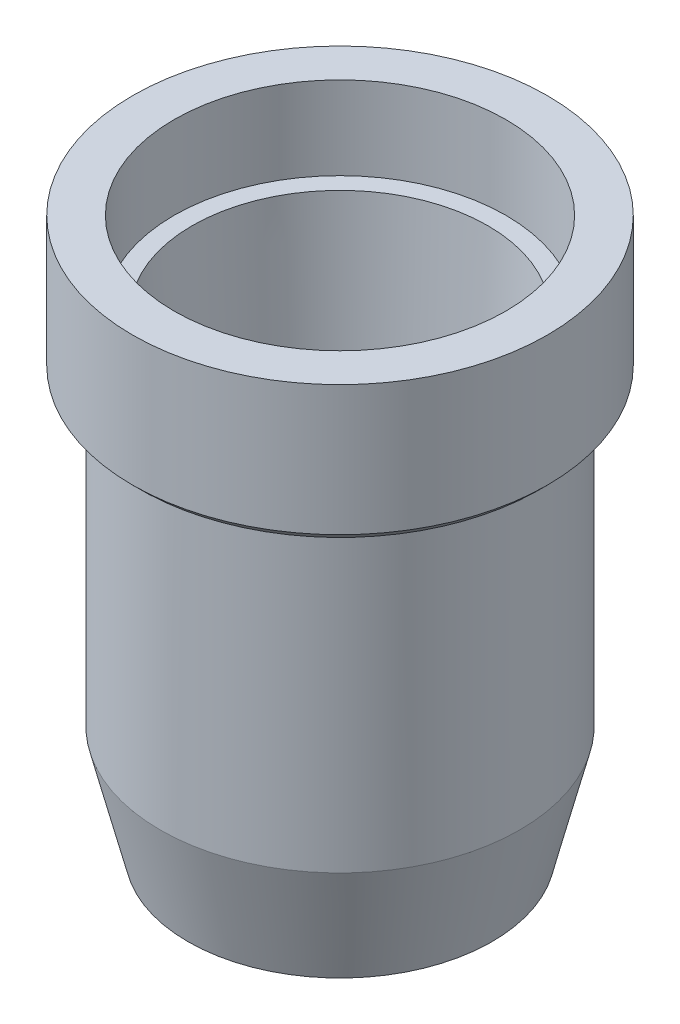
from build123d import *

# Parameters (mm, degrees)
SKETCH1_R           = 7.5
SKETCH1_R_2         = 4.75
BOSS_EXTRUDE1_DEPTH = 20
SKETCH2_R           = 6
CUT_EXTRUDE1_DEPTH  = 3
SKETCH3_OUTSIDE_W   = 22.83
SKETCH3_OUTSIDE_H   = 22.83
SKETCH3_OUTSIDE_R   = 6.5
CUT_EXTRUDE2_DEPTH  = 15
CHAMFER1_SIZE       = 0.6
CHAMFER1_SIZE2      = 10
CHAMFER2_SIZE       = 0.3
CHAMFER3_SIZE       = 4
CHAMFER3_SIZE2      = 1


with BuildPart() as part:
    # Sketch1 → Boss-Extrude1 (new body)
    with BuildSketch(Plane(origin=(0, 0, 0), x_dir=(1, 0, 0), z_dir=(0, 1, 0))):
        with Locations(Location((0, 0, 0), (0, 0, 270))):
            Circle(SKETCH1_R)
        with Locations(Location((0, 0, 0), (0, 0, 270))):
            Circle(SKETCH1_R_2, mode=Mode.SUBTRACT)
    extrude(amount=BOSS_EXTRUDE1_DEPTH)

    # Sketch2 → Cut-Extrude1 (cut)
    with BuildSketch(Plane(origin=(0, 20, 0), x_dir=(1, 0, 0), z_dir=(0, 1, 0))):
        with Locations(Location((0, 0, 0), (0, 0, 270))):
            Circle(SKETCH2_R)
    extrude(amount=-CUT_EXTRUDE1_DEPTH, mode=Mode.SUBTRACT)

    # Sketch3 outside → Cut-Extrude2 (cut)
    with BuildSketch(Plane.XZ):
        Rectangle(SKETCH3_OUTSIDE_W, SKETCH3_OUTSIDE_H)
        with Locations(Location((0, 0, 0), (0, 0, 270))):
            Circle(SKETCH3_OUTSIDE_R, mode=Mode.SUBTRACT)
    extrude(amount=-CUT_EXTRUDE2_DEPTH, mode=Mode.SUBTRACT)

    # Chamfer1
    chamfer1_edges = [part.edges().sort_by_distance(p)[0] for p in [
        (0, 17, -4.75),
    ]]
    chamfer1_side = [part.faces().sort_by_distance(p)[0] for p in [
        (0, 17, -5.830294373),
    ]]
    chamfer(chamfer1_edges, length=CHAMFER1_SIZE, length2=CHAMFER1_SIZE2, reference=chamfer1_side[0])

    # Chamfer2
    chamfer2_edges = [part.edges().sort_by_distance(p)[0] for p in [
        (0, 15, -7.5),
    ]]
    chamfer(chamfer2_edges, length=CHAMFER2_SIZE)

    # Chamfer3
    chamfer3_edges = [part.edges().sort_by_distance(p)[0] for p in [
        (0, 0, 6.5),
    ]]
    chamfer3_side = [part.faces().sort_by_distance(p)[0] for p in [
        (0, 7.5, 6.5),
    ]]
    chamfer(chamfer3_edges, length=CHAMFER3_SIZE, length2=CHAMFER3_SIZE2, reference=chamfer3_side[0])


solid = part.part
